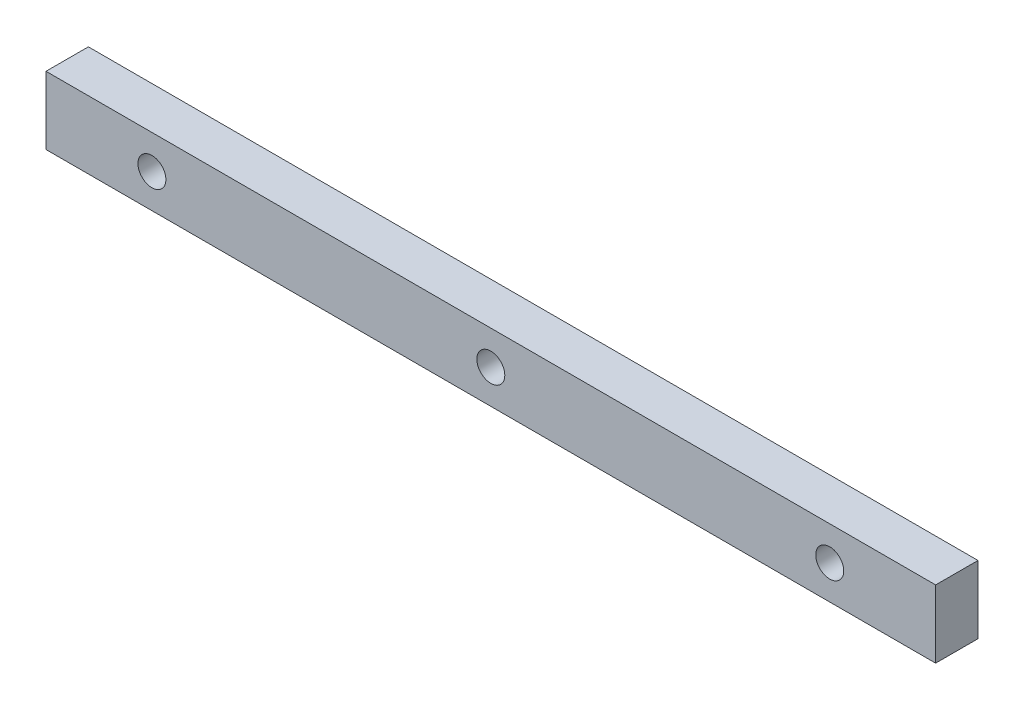
SolidWorks part; units mm, degrees
ref_plane "Front Plane" through (0, 0, 0) normal (0, 0, 1) x (1, 0, 0)
ref_plane "Top Plane" through (0, 0, 0) normal (0, 1, 0) x (1, 0, 0)
ref_plane "Right Plane" through (0, 0, 0) normal (1, 0, 0) x (0, 0, -1)
other "Configuration Table"
sketch "Sketch1" plane through (0, 0, 0) normal (0, 0, 1) x (1, 0, 0)
  line L1 (-52.5, 4) -> (52.5, 4)
  line L2 (-52.5, 4) -> (-52.5, -4)
  line L3 (-52.5, -4) -> (52.5, -4)
  line L4 (52.5, 4) -> (52.5, -4)
  line L5 (-52.5, 4) -> (52.5, -4) construction
  line L6 (-52.5, -4) -> (52.5, 4) construction
  point P0 (0, 0)
extrude "Boss-Extrude1" add sketch "Sketch1" along normal blind 5
sketch "Sketch2" plane through (0, 0, 5) normal (0, 0, 1) x (1, 0, 0)
  circle A0 centre (0, 0) radius 2
  circle A1 centre (-40, 0) radius 2
  circle A2 centre (40, 0) radius 2
  dimension "D1" = 40
  dimension "D2" = 40
hole_wizard "M4 Tapped Hole2" positions "Sketch6" profile "Sketch5" tap size "M4" standard "GB" end condition through all
sketch "Sketch6" plane through (0, 0, 5) normal (0, 0, 1) x (1, 0, 0)
  point P0 (-40, 0)
  point P3 (0, 0)
  point P6 (40, 0)
sketch "Sketch5" plane through (-40, 0, 5) normal (1, 0, 0) x (0, -1, 0)
  line L0 (0, 0) -> (0, 5)
  line L1 (0, 5) -> (1.65, 5)
  line L2 (1.65, 5) -> (1.65, 0)
  line L5 (1.65, 0) -> (0, 0)
  line L11 (0, -6.35) -> (0, 107.95) construction
  dimension "通孔螺纹孔钻头直径" = 3.3
  dimension "通孔螺纹孔钻头深度" = 5
cosmetic thread "Cosmetic Thread1"
cosmetic thread "Cosmetic Thread4"
cosmetic thread "Cosmetic Thread5"
